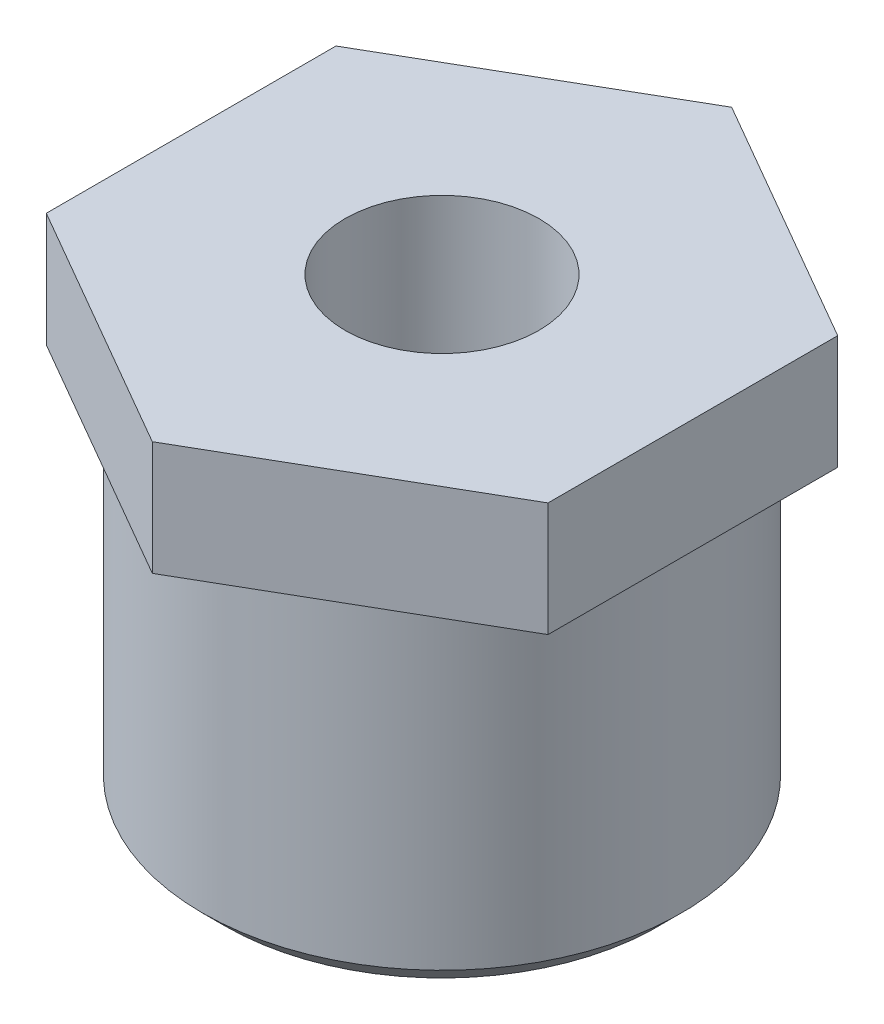
from build123d import *

# Parameters (mm, degrees)
BOSS_EXTRUDE1_DEPTH = 20
SKETCH3_OUTSIDE_W   = 31.822
SKETCH3_OUTSIDE_H   = 35.226
SKETCH3_OUTSIDE_R   = 10.5
CUT_EXTRUDE1_DEPTH  = 15
CHAMFER1_SIZE       = 1
M10_TAPPED_HOLE1_D  = 8.5


with BuildPart() as part:
    # Sketch1 → Boss-Extrude1 (new body)
    with BuildSketch(Plane(origin=(0, 0, 0), x_dir=(1, 0, 0), z_dir=(0, 1, 0))):
        Polygon((11, -6.350852961), (11, 6.350852961), (0, 12.701705922), (-11, 6.350852961), (-11, -6.350852961), (0, -12.701705922), align=None)
    extrude(amount=BOSS_EXTRUDE1_DEPTH)

    # Sketch3 outside → Cut-Extrude1 (cut)
    with BuildSketch(Plane.XZ):
        Rectangle(SKETCH3_OUTSIDE_W, SKETCH3_OUTSIDE_H)
        with Locations(Location((0, 0, 0), (0, 0, 270))):
            Circle(SKETCH3_OUTSIDE_R, mode=Mode.SUBTRACT)
    extrude(amount=-CUT_EXTRUDE1_DEPTH, mode=Mode.SUBTRACT)

    # Chamfer1
    chamfer1_edges = [part.edges().sort_by_distance(p)[0] for p in [
        (0, 0, 10.5),
    ]]
    chamfer(chamfer1_edges, length=CHAMFER1_SIZE)

    # M10 Tapped Hole1 (through all)
    with Locations(Plane.ZX.offset(20)):
        with Locations((0, 0)):
            Hole(M10_TAPPED_HOLE1_D / 2)


solid = part.part
